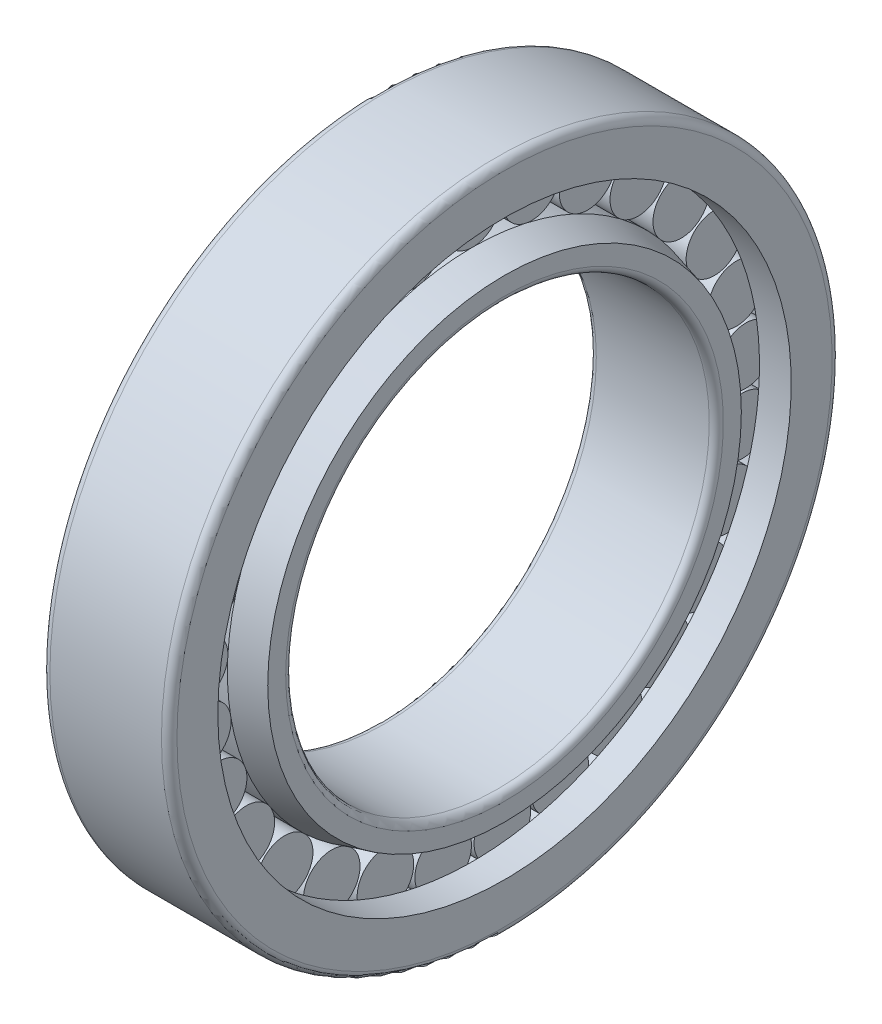
from build123d import *

# Parameters (mm, degrees)
SKETCH2_W               = 9
SKETCH2_H               = 4.01
CIRCULAR_PATTERN1_COUNT = 29
FILLET1_R               = 1.1
FILLET2_R               = 1


with BuildPart() as part:
    # Sketch1 → Revolve1 (revolve)
    with BuildSketch(Plane.XY, mode=Mode.PRIVATE) as revolve1_sk:
        Polygon((-9, 30), (9, 30), (9, 33.544228634), (4.5, 34.75), (-4.5, 34.75), (-9, 33.544228634), align=None)
    revolve(revolve1_sk.sketch.rotate(Axis((-10.137871204, 0, 0), (1, 0, 0)), 90), axis=Axis((-10.137871204, 0, 0), (1, 0, 0)))

    # Sketch2 → Revolve2 (revolve)
    with BuildSketch(Plane.XY):
        with Locations((0, 36.745)):
            Rectangle(SKETCH2_W, SKETCH2_H)
    revolve2 = revolve(axis=Axis((-7.422783257, 38.75, 0), (1, 0, 0)))

    # Sketch3 → Revolve3 (revolve)
    with BuildSketch(Plane.XY, mode=Mode.PRIVATE) as revolve3_sk:
        Polygon((-9, 47.5), (9, 47.5), (9, 40.6125), (4.49, 40.6125), (4.49, 42.75), (-4.49, 42.75), (-4.49, 40.6125), (-9, 40.6125), align=None)
    revolve(revolve3_sk.sketch.rotate(Axis((-9.082213196, 0, 0), (1, 0, 0)), 90), axis=Axis((-9.082213196, 0, 0), (1, 0, 0)))

    # Circular-Pattern1: Revolve2 ×29 about axis
    circular_pattern1_axis = Axis((0, 0, 0), (1, 0, 0))
    for i in range(1, CIRCULAR_PATTERN1_COUNT):
        add(revolve2.rotate(circular_pattern1_axis, i * 360 / CIRCULAR_PATTERN1_COUNT))

    # Fillet1
    fillet1_edges = [part.edges().sort_by_distance(p)[0] for p in [
        (-9, 0, -47.5),
        (9, 0, -47.5),
    ]]
    fillet(fillet1_edges, radius=FILLET1_R)

    # Fillet2
    fillet2_edges = [part.edges().sort_by_distance(p)[0] for p in [
        (9, 0, -30),
        (-9, 0, -30),
    ]]
    fillet(fillet2_edges, radius=FILLET2_R)


solid = part.part
